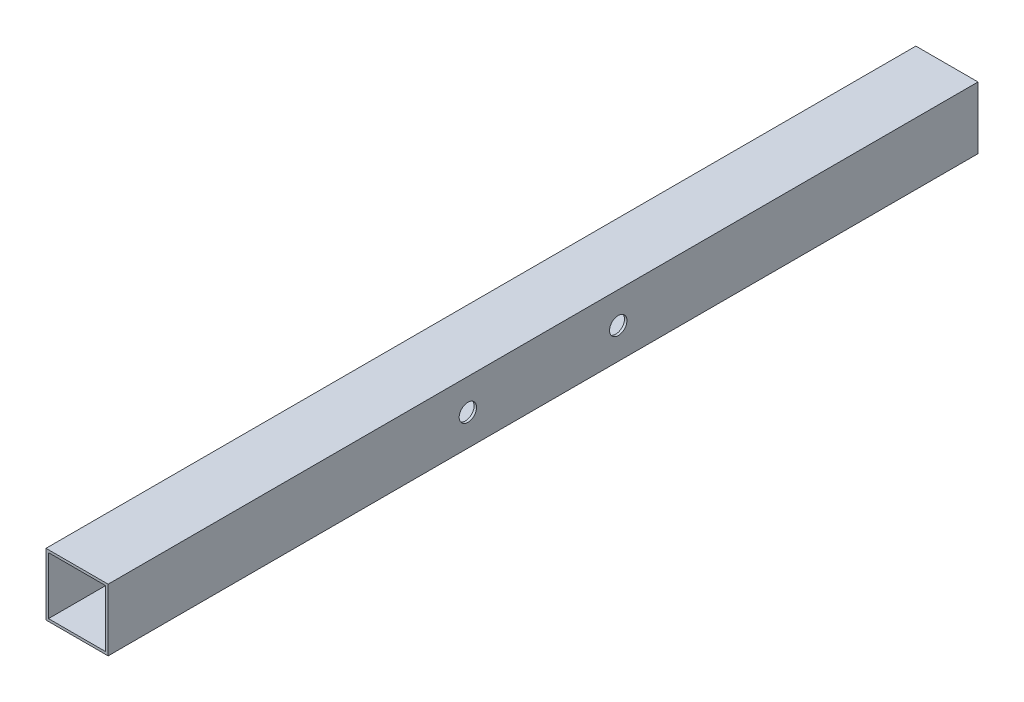
from build123d import *

# Parameters (mm, degrees)
SKETCH1_W           = 50
SKETCH1_H           = 50
SKETCH1_W_2         = 46
SKETCH1_H_2         = 46
BOSS_EXTRUDE1_DEPTH = 700
SKETCH2_R           = 7
CUT_EXTRUDE1_DEPTH  = 703.228595259


with BuildPart() as part:
    # Sketch1 → Boss-Extrude1 (new body)
    with BuildSketch(Plane.XY):
        Rectangle(SKETCH1_W, SKETCH1_H)
        Rectangle(SKETCH1_W_2, SKETCH1_H_2, mode=Mode.SUBTRACT)
    extrude(amount=BOSS_EXTRUDE1_DEPTH)

    # Sketch2 → Cut-Extrude1 (cut, through all)
    with BuildSketch(Plane.ZY.offset(25)):
        with Locations((289.5, 0)):
            Circle(SKETCH2_R)
        with Locations(Location((410.5, 0, 0), (0, 0, 180))):
            Circle(SKETCH2_R)
    extrude(amount=-CUT_EXTRUDE1_DEPTH, mode=Mode.SUBTRACT)


solid = part.part
